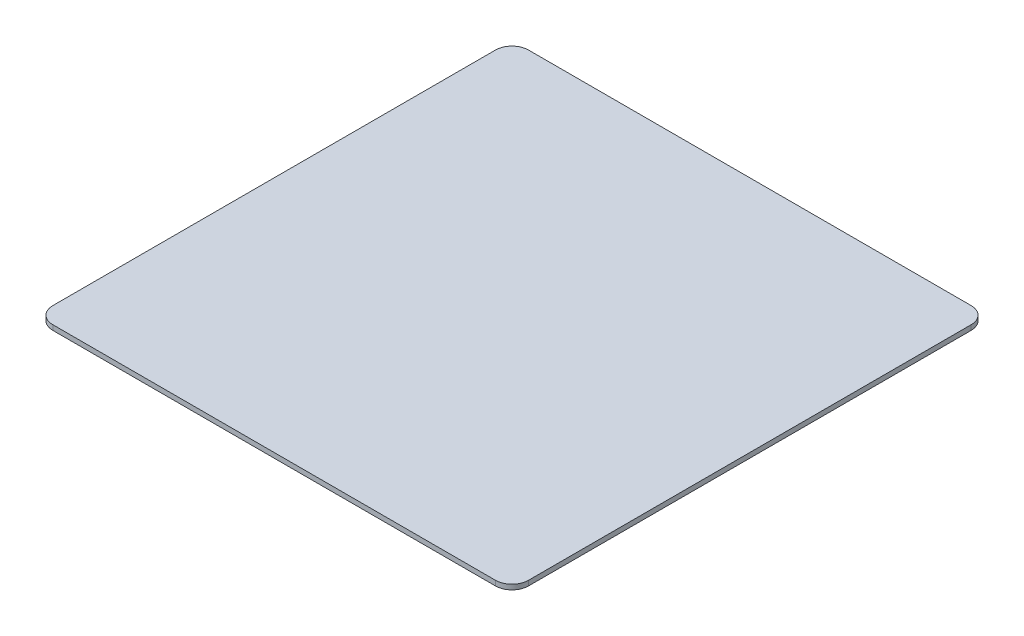
from build123d import *

# Parameters (mm, degrees)
BOSS_EXTRUDE1_DEPTH = 3


with BuildPart() as part:
    # Sketch1 → Boss-Extrude1 (new body)
    with BuildSketch(Plane(origin=(0, 0, 0), x_dir=(1, 0, 0), z_dir=(0, 1, 0))):
        with BuildLine():
            Line((-134, -144), (134, -144))
            ThreePointArc((134, -144), (141.071067812, -141.071067812), (144, -134))
            Line((144, -134), (144, 134))
            ThreePointArc((144, 134), (141.071067812, 141.071067812), (134, 144))
            Line((134, 144), (-134, 144))
            ThreePointArc((-134, 144), (-141.071067812, 141.071067812), (-144, 134))
            Line((-144, 134), (-144, -134))
            ThreePointArc((-144, -134), (-141.071067812, -141.071067812), (-134, -144))
        make_face()
    extrude(amount=BOSS_EXTRUDE1_DEPTH)


solid = part.part
